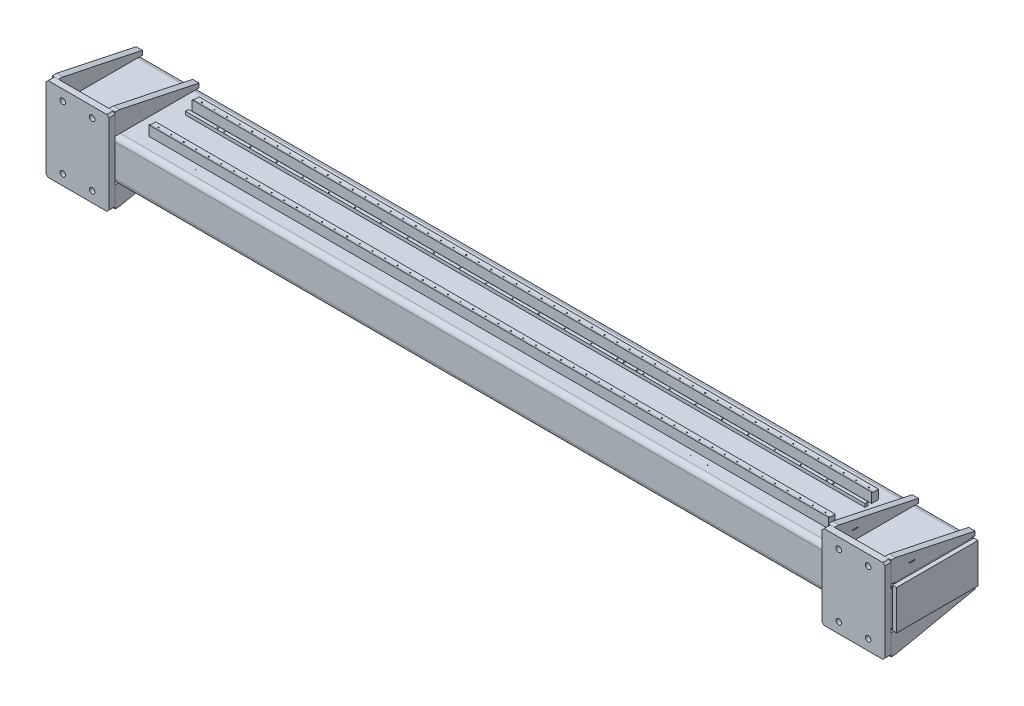
SolidWorks part; units mm, degrees
material "普通碳钢"
ref_plane "前视基准面" through (0, 0, 0) normal (0, 0, 1) x (1, 0, 0)
ref_plane "上视基准面" through (0, 0, 0) normal (0, 1, 0) x (1, 0, 0)
ref_plane "右视基准面" through (0, 0, 0) normal (1, 0, 0) x (0, 0, -1)
sketch "草图1" plane through (0, 0, 0) normal (0, 0, 1) x (1, 0, 0)
  line L0 (-2000, 0) -> (2000, 0)
  point P4 (0, 0)
  dimension "D1" = 4000
other "Gb／6728-1986矩形空心型钢 400 X 200 X 12(1)"
ref_plane "基准面1" through (-2000, 0, 0) normal (1, 0, 0) x (0, 1, 0)
sketch "Sketch13" plane through (-2000, 0, 0) normal (1, 0, 0) x (0, 1, 0)
  line L0 (-76, -188) -> (76, -188)
  line L1 (-88, -176) -> (-88, 176)
  line L2 (76, 188) -> (-76, 188)
  line L3 (88, 176) -> (88, -176)
  line L4 (-76, -200) -> (76, -200)
  line L5 (-100, -176) -> (-100, 176)
  line L6 (76, 200) -> (-76, 200)
  line L7 (100, 176) -> (100, -176)
  arc A0 (100, 176) -> (76, 200) centre (76, 176) ccw
  arc A1 (76, -200) -> (100, -176) centre (76, -176) ccw
  arc A2 (-100, -176) -> (-76, -200) centre (-76, -176) ccw
  arc A3 (-76, 200) -> (-100, 176) centre (-76, 176) ccw
  arc A4 (-76, 188) -> (-88, 176) centre (-76, 176) ccw
  arc A5 (88, 176) -> (76, 188) centre (76, 176) ccw
  arc A6 (76, -188) -> (88, -176) centre (76, -176) ccw
  arc A7 (-88, -176) -> (-76, -188) centre (-76, -176) ccw
  point P0 (0, 200)
  point P1 (100, 0)
  point P2 (0, -200)
  point P3 (-100, 0)
  point P4 (-100, 200)
  point P5 (100, 200)
  point P6 (100, -200)
  point P7 (-100, -200)
  point P8 (0, 0)
  point P33 (0, 0)
  dimension "D1" = 24
  dimension "Thickness" = 12
  dimension "V_leg" = 400
  dimension "H_leg" = 200
sketch "草图5" plane through (0, 0, 200) normal (0, 0, 1) x (1, 0, 0)
  line L1 (-2000, 200) -> (-1700, 200)
  line L2 (-2000, 200) -> (-2000, -200)
  line L3 (-2000, -200) -> (-1700, -200)
  line L4 (-1700, 200) -> (-1700, -200)
  line L5 (0, 0) -> (0, 871.3607) construction
  line L6 (1700, 200) -> (1700, -200)
  line L7 (2000, -200) -> (1700, -200)
  line L8 (2000, 200) -> (2000, -200)
  line L9 (2000, 200) -> (1700, 200)
  line L10 (-2000, 76) -> (-2000, -76) construction
  line L11 (-1708.2298, 0) -> (-1072.1505, 0) construction
  line L12 (-2000, 0) -> (2000, 0) construction
  dimension "D1" = 300
  dimension "D2" = 400
extrude "凸台-拉伸1" add sketch "草图5" along normal blind 30 separate body
sketch "草图6" plane through (-2000, 0, 0) normal (-1, 0, 0) x (0, 0, 1)
  line L0 (-200, 100) -> (-200, 120)
  line L1 (-200, 120) -> (180, 200)
  line L2 (180, 200) -> (200, 200)
  line L3 (200, 200) -> (200, 100)
  line L4 (200, 200) -> (200, -200) construction
  line L5 (200, 100) -> (-200, 100)
  line L6 (-176, 100) -> (176, 100) construction
  line L7 (-200, -76) -> (-200, 76) construction
  dimension "D1" = 20
  dimension "D2" = 20
extrude "凸台-拉伸2" add sketch "草图6" against normal blind 30 separate body
other "顶端盖1" parameters "D1"=20, "D2"=3, "D3"=3
other "顶端盖2" parameters "D1"=20, "D2"=3, "D3"=3
ref_plane "基准面2" through (-1850, 0, 0) normal (1, 0, 0) x (0, 0, -1)
mirror "镜向3" about plane through (-1850, 0, 0) normal (1, 0, 0) of bodies 109
mirror "镜向4" about plane through (0, 0, 0) normal (0, 1, 0) of bodies 113 109
mirror "镜向5" about plane through (0, 0, 0) normal (1, 0, 0) of bodies 115 114 109 113
chamfer "倒角1" distance 10 angle 45 4 edges at (-2000, 200, 215) (-1700, 200, 215) (-1700, -200, 215) (-2000, -200, 215)
chamfer "倒角2" distance 10 angle 45 4 edges at (2000, 200, 215) (2000, -200, 215) (1700, -200, 215) (1700, 200, 215)
sketch "草图7" plane through (0, 100, 0) normal (0, 1, 0) x (1, 0, 0)
  line L0 (0, 0) -> (0, -385.6648) construction
  line L1 (-1620, 120) -> (1620, 120)
  line L2 (-1620, 120) -> (-1620, 87)
  line L3 (-1620, 87) -> (1620, 87)
  line L4 (1620, 120) -> (1620, 87)
  line L5 (2000, 200) -> (-2000, 200) construction
  line L7 (0, 0) -> (-2193.4981, 0) construction
  line L8 (1620, -120) -> (1620, -87)
  line L9 (-1620, -120) -> (1620, -120)
  line L10 (-1620, -120) -> (-1620, -87)
  line L11 (-1620, -87) -> (1620, -87)
  dimension "D1" = 80
  dimension "D2" = 33
  dimension "D3" = 3240
extrude "凸台-拉伸3" add sketch "草图7" along normal blind 47 separate body
sketch "草图8" plane through (-1620, 0, 0) normal (-1, 0, 0) x (0, 0, 1)
  line L0 (-87, 147) -> (-87, 100) construction
  line L1 (-120, 147) -> (-92, 147)
  line L2 (-120, 147) -> (-120, 143)
  line L3 (-120, 143) -> (-92, 143)
  line L4 (-92, 147) -> (-92, 143)
  line L5 (120, 147) -> (120, 100) construction
  line L6 (87, 147) -> (115, 147)
  line L7 (87, 147) -> (87, 143)
  line L8 (87, 143) -> (115, 143)
  line L9 (115, 147) -> (115, 143)
  dimension "D1" = 4
  dimension "D2" = 5
  dimension "D3" = 5
extrude "切除-拉伸1" cut sketch "草图8" against normal through all
sketch "草图11" plane through (0, 143, 0) normal (0, 1, 0) x (1, 0, 0)
  line L0 (-1620, 120) -> (-1620, 92) construction
  line L1 (1620, 120) -> (-1620, 120) construction
  line L2 (0, 0) -> (310.4393, 0) construction
  point P0 (-1590, 103.5)
  point P20 (-1530, 103.5)
  point P21 (-1470, 103.5)
  point P22 (-1410, 103.5)
  point P23 (-1350, 103.5)
  point P24 (-1290, 103.5)
  point P25 (-1230, 103.5)
  point P26 (-1170, 103.5)
  point P27 (-1110, 103.5)
  point P28 (-1050, 103.5)
  point P29 (-990, 103.5)
  point P30 (-930, 103.5)
  point P31 (-870, 103.5)
  point P32 (-810, 103.5)
  point P33 (-750, 103.5)
  point P34 (-690, 103.5)
  point P35 (-630, 103.5)
  point P36 (-570, 103.5)
  point P37 (-510, 103.5)
  point P38 (-450, 103.5)
  point P39 (-390, 103.5)
  point P40 (-330, 103.5)
  point P41 (-270, 103.5)
  point P42 (-210, 103.5)
  point P43 (-150, 103.5)
  point P44 (-90, 103.5)
  point P45 (-30, 103.5)
  point P46 (30, 103.5)
  point P47 (90, 103.5)
  point P48 (150, 103.5)
  point P49 (210, 103.5)
  point P50 (270, 103.5)
  point P51 (330, 103.5)
  point P52 (390, 103.5)
  point P53 (450, 103.5)
  point P54 (510, 103.5)
  point P55 (570, 103.5)
  point P56 (630, 103.5)
  point P57 (690, 103.5)
  point P58 (750, 103.5)
  point P59 (810, 103.5)
  point P60 (870, 103.5)
  point P61 (930, 103.5)
  point P62 (990, 103.5)
  point P63 (1050, 103.5)
  point P64 (1110, 103.5)
  point P65 (1170, 103.5)
  point P66 (1230, 103.5)
  point P67 (1290, 103.5)
  point P68 (1350, 103.5)
  point P69 (1410, 103.5)
  point P70 (1470, 103.5)
  point P71 (1530, 103.5)
  point P72 (1590, 103.5)
  dimension "D1" = 30
  dimension "D2" = 16.5
  dimension "D4" = 60
  dimension "D3" = 54
hole_wizard "M6 螺纹孔1" positions "草图11" profile "草图10" tap size "M6" standard "GB"
sketch "草图10" plane through (-1590, 143, -103.5) normal (1, 0, 0) x (0, 0, 1)
  line L0 (0, 0) -> (0, 16.5022)
  line L1 (0, 16.5022) -> (2.5, 15)
  line L2 (2.5, 15) -> (2.5, 0)
  line L5 (2.5, 0) -> (0, 0)
  line L10 (0, 16.5022) -> (-2.5, 15) construction
  line L11 (0, -6.35) -> (0, 107.95) construction
  dimension "螺纹孔钻头直径" = 5
  dimension "螺纹孔钻头深度" = 15
  dimension "导头角度" = 118
cosmetic thread "孔螺纹线1"
cosmetic thread "孔螺纹线2"
cosmetic thread "孔螺纹线3"
cosmetic thread "孔螺纹线4"
cosmetic thread "孔螺纹线5"
cosmetic thread "孔螺纹线6"
cosmetic thread "孔螺纹线7"
cosmetic thread "孔螺纹线8"
cosmetic thread "孔螺纹线9"
cosmetic thread "孔螺纹线10"
cosmetic thread "孔螺纹线11"
cosmetic thread "孔螺纹线12"
cosmetic thread "孔螺纹线13"
cosmetic thread "孔螺纹线14"
cosmetic thread "孔螺纹线15"
cosmetic thread "孔螺纹线16"
cosmetic thread "孔螺纹线17"
cosmetic thread "孔螺纹线18"
cosmetic thread "孔螺纹线19"
cosmetic thread "孔螺纹线20"
cosmetic thread "孔螺纹线21"
cosmetic thread "孔螺纹线22"
cosmetic thread "孔螺纹线23"
cosmetic thread "孔螺纹线24"
cosmetic thread "孔螺纹线25"
cosmetic thread "孔螺纹线26"
cosmetic thread "孔螺纹线27"
cosmetic thread "孔螺纹线28"
cosmetic thread "孔螺纹线29"
cosmetic thread "孔螺纹线30"
cosmetic thread "孔螺纹线31"
cosmetic thread "孔螺纹线32"
cosmetic thread "孔螺纹线33"
cosmetic thread "孔螺纹线34"
cosmetic thread "孔螺纹线35"
cosmetic thread "孔螺纹线36"
cosmetic thread "孔螺纹线37"
cosmetic thread "孔螺纹线38"
cosmetic thread "孔螺纹线39"
cosmetic thread "孔螺纹线40"
cosmetic thread "孔螺纹线41"
cosmetic thread "孔螺纹线42"
cosmetic thread "孔螺纹线43"
cosmetic thread "孔螺纹线44"
cosmetic thread "孔螺纹线45"
cosmetic thread "孔螺纹线46"
cosmetic thread "孔螺纹线47"
cosmetic thread "孔螺纹线48"
cosmetic thread "孔螺纹线49"
cosmetic thread "孔螺纹线50"
cosmetic thread "孔螺纹线51"
cosmetic thread "孔螺纹线52"
cosmetic thread "孔螺纹线53"
cosmetic thread "孔螺纹线54"
mirror "镜向6" about plane through (0, 0, 0) normal (0, 0, 1) of "M6 螺纹孔1"
sketch "草图14" plane through (0, 0, 200) normal (0, 0, -1) x (-1, 0, 0)
  line L0 (1710, 200) -> (1990, 200) construction
  line L1 (2000, 190) -> (2000, -190) construction
  line L2 (2020, 0) -> (-2030.2689, 0) construction
  line L3 (2020, 94) -> (2020, -94) construction
  line L5 (1850, 200) -> (1850, -200.5459) construction
  line L6 (1710, 200) -> (1990, 200) construction
  line L7 (1850, 16.5) -> (1850, -16.5) construction
  line L9 (0, 0) -> (0, 682.3261) construction
  line L11 (-1850, 200) -> (-1850, -200.5459) construction
  line L12 (-2020, 0) -> (2030.2689, 0) construction
  point P0 (1920, 150)
  point P24 (1780, 150)
  point P25 (1780, -150)
  point P26 (1920, -150)
  point P34 (-1920, -150)
  point P35 (-1780, -150)
  point P36 (-1780, 150)
  point P37 (-1920, 150)
  dimension "D1" = 50
  dimension "D2" = 80
hole_wizard "M24 间隙孔1" positions "草图14" profile "草图13" hole size "M24" standard "GB" end condition through all
sketch "草图13" plane through (-1920, 150, 200) normal (1, 0, 0) x (0, 1, 0)
  line L0 (0, 0) -> (0, 30)
  line L1 (0, 30) -> (13, 30)
  line L2 (13, 30) -> (13, 0)
  line L5 (13, 0) -> (0, 0)
  line L11 (0, -6.35) -> (0, 107.95) construction
  dimension "通孔孔直径" = 26
  dimension "通孔孔深度" = 30
sketch "草图15" plane through (-1620, 0, 0) normal (-1, 0, 0) x (0, 0, 1)
  line L0 (-200, 100) -> (200, 100) construction
  line L1 (-55, 100) -> (-70, 100)
  line L2 (-55, 100) -> (-55, 116)
  line L3 (-55, 116) -> (-70, 116)
  line L4 (-70, 100) -> (-70, 116)
  line L5 (0, 0) -> (0, 180.8221) construction
  dimension "D1" = 16
  dimension "D2" = 70
  dimension "D3" = 15
extrude "凸台-拉伸4" add sketch "草图15" against normal up to surface (3240 mm away) separate body up to face at (1620, 130, -99.6667)
sketch "草图18" plane through (0, 116, 0) normal (0, 1, 0) x (1, 0, 0)
  point P0 (-1442.5, 61.745)
  point P3 (-1317.3781, 61.745)
  point P5 (-1192.5, 61.745)
  point P8 (-1067.5, 61.745)
  point P11 (-942.5, 61.745)
  point P14 (-817.5, 61.745)
  point P17 (-692.5, 61.745)
  point P20 (-567.5, 61.745)
  point P23 (-442.5, 61.745)
  point P26 (-317.5, 61.745)
  point P29 (-192.5, 61.745)
  point P32 (-67.5, 61.745)
  point P35 (57.5, 61.745)
  point P38 (182.5, 61.745)
  point P41 (307.5, 61.745)
  point P44 (432.5, 61.745)
  point P47 (557.5, 61.745)
  point P50 (682.5, 61.745)
  point P53 (807.5, 61.745)
  point P56 (932.5, 61.745)
  point P59 (1057.5, 61.745)
  point P62 (1182.5, 61.745)
  point P65 (1307.5, 61.745)
  point P68 (1432.5, 61.745)
hole_wizard "M6 螺纹孔2" positions "草图18" profile "草图17" tap size "M6" standard "GB"
sketch "草图17" plane through (-1442.5, 116, -61.745) normal (1, 0, 0) x (0, 0, 1)
  line L0 (0, 0) -> (0, 16.5022)
  line L1 (0, 16.5022) -> (2.5, 15)
  line L2 (2.5, 15) -> (2.5, 0)
  line L5 (2.5, 0) -> (0, 0)
  line L10 (0, 16.5022) -> (-2.5, 15) construction
  line L11 (0, -6.35) -> (0, 107.95) construction
  dimension "螺纹孔钻头直径" = 5
  dimension "螺纹孔钻头深度" = 15
  dimension "导头角度" = 118
cosmetic thread "孔螺纹线55"
cosmetic thread "孔螺纹线56"
cosmetic thread "孔螺纹线57"
cosmetic thread "孔螺纹线58"
cosmetic thread "孔螺纹线59"
cosmetic thread "孔螺纹线60"
cosmetic thread "孔螺纹线61"
cosmetic thread "孔螺纹线62"
cosmetic thread "孔螺纹线63"
cosmetic thread "孔螺纹线64"
cosmetic thread "孔螺纹线65"
cosmetic thread "孔螺纹线66"
cosmetic thread "孔螺纹线67"
cosmetic thread "孔螺纹线68"
cosmetic thread "孔螺纹线69"
cosmetic thread "孔螺纹线70"
cosmetic thread "孔螺纹线71"
cosmetic thread "孔螺纹线72"
cosmetic thread "孔螺纹线73"
cosmetic thread "孔螺纹线74"
cosmetic thread "孔螺纹线75"
cosmetic thread "孔螺纹线76"
cosmetic thread "孔螺纹线77"
cosmetic thread "孔螺纹线78"
sketch "草图21" plane through (0, 116, 0) normal (0, 1, 0) x (1, 0, 0)
  point P0 (-1473.3, 61.745)
  point P3 (463.3, 61.745)
  point P6 (526.7, 61.745)
  point P9 (1463.3, 61.745)
hole_wizard "Ø6.0mm 暗销孔1" positions "草图21" profile "草图20" hole size "Ø6.0" standard "GB"
sketch "草图20" plane through (-1473.3, 116, -61.745) normal (1, 0, 0) x (0, 0, 1)
  line L0 (0, 0) -> (0, 16.8026)
  line L1 (0, 16.8026) -> (3, 15)
  line L2 (3, 15) -> (3, 0)
  line L5 (3, 0) -> (0, 0)
  line L10 (0, 16.8026) -> (-3, 15) construction
  line L11 (0, -6.35) -> (0, 107.95) construction
  dimension "孔直径" = 6
  dimension "孔深度" = 15
  dimension "导头角度" = 118
sketch "草图24" plane through (0, 0, -200) normal (0, 0, -1) x (-1, 0, 0)
  point P0 (-1850, 62.5)
  point P3 (-1815, 62.5)
  point P6 (-1850, -62.5)
  point P9 (-1815, -62.5)
hole_wizard "M8 螺纹孔1" positions "草图24" profile "草图23" tap size "M8" standard "GB" end condition up to next
sketch "草图23" plane through (1850, 62.5, -200) normal (1, 0, 0) x (0, 1, 0)
  line L0 (0, 0) -> (0, 12.001)
  line L1 (0, 12.001) -> (3.4, 12.001)
  line L2 (3.4, 12.001) -> (3.4, 0)
  line L5 (3.4, 0) -> (0, 0)
  line L11 (0, -6.35) -> (0, 107.95) construction
  dimension "通孔螺纹孔钻头直径" = 6.8
  dimension "通孔螺纹孔钻头深度" = 12.001
cosmetic thread "孔螺纹线79"
cosmetic thread "孔螺纹线80"
cosmetic thread "孔螺纹线81"
cosmetic thread "孔螺纹线82"
sketch "草图27" plane through (0, 100, 0) normal (0, 1, 0) x (1, 0, 0)
  point P0 (-1450, -146)
  point P3 (-1370, -146)
  point P6 (990, -146)
  point P9 (1070, -146)
hole_wizard "M3 螺纹孔1" positions "草图27" profile "草图26" tap size "M3" standard "GB" end condition up to next
sketch "草图26" plane through (-1450, 100, 146) normal (1, 0, 0) x (0, 0, 1)
  line L0 (0, 0) -> (0, 12.001)
  line L1 (0, 12.001) -> (1.25, 12.001)
  line L2 (1.25, 12.001) -> (1.25, 0)
  line L5 (1.25, 0) -> (0, 0)
  line L11 (0, -6.35) -> (0, 107.95) construction
  dimension "通孔螺纹孔钻头直径" = 2.5
  dimension "通孔螺纹孔钻头深度" = 12.001
cosmetic thread "孔螺纹线83"
cosmetic thread "孔螺纹线84"
cosmetic thread "孔螺纹线85"
cosmetic thread "孔螺纹线86"
